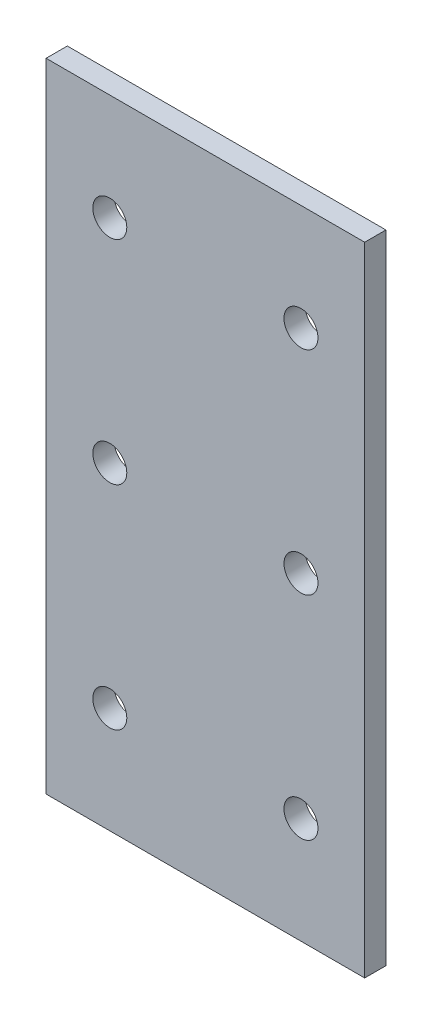
SolidWorks part; units mm, degrees
ref_plane "Front Plane" through (0, 0, 0) normal (0, 0, 1) x (1, 0, 0)
ref_plane "Top Plane" through (0, 0, 0) normal (0, 1, 0) x (1, 0, 0)
ref_plane "Right Plane" through (0, 0, 0) normal (1, 0, 0) x (0, 0, -1)
sketch "Sketch1" plane through (0, 0, 0) normal (0, 0, 1) x (1, 0, 0)
  line L0 (0, 0) -> (0, 101.2477) construction
  line L1 (75, 150) -> (-75, 150)
  line L2 (75, 150) -> (75, -150)
  line L3 (75, -150) -> (-75, -150)
  line L4 (-75, 150) -> (-75, -150)
  line L5 (75, 150) -> (-75, -150) construction
  line L6 (75, -150) -> (-75, 150) construction
  circle A0 centre (-45, 100) radius 8
  circle A2 centre (-45, 0) radius 8
  circle A3 centre (-45, -100) radius 8
  circle A4 centre (45, -100) radius 8
  circle A5 centre (45, 0) radius 8
  circle A6 centre (45, 100) radius 8
  point P0 (0, 0)
  dimension "D1" = 16
  dimension "D2" = 100
  dimension "D3" = 100
  dimension "D4" = 45
  dimension "D5" = 150
  dimension "D6" = 300
extrude "Boss-Extrude1" add sketch "Sketch1" along normal blind 10
